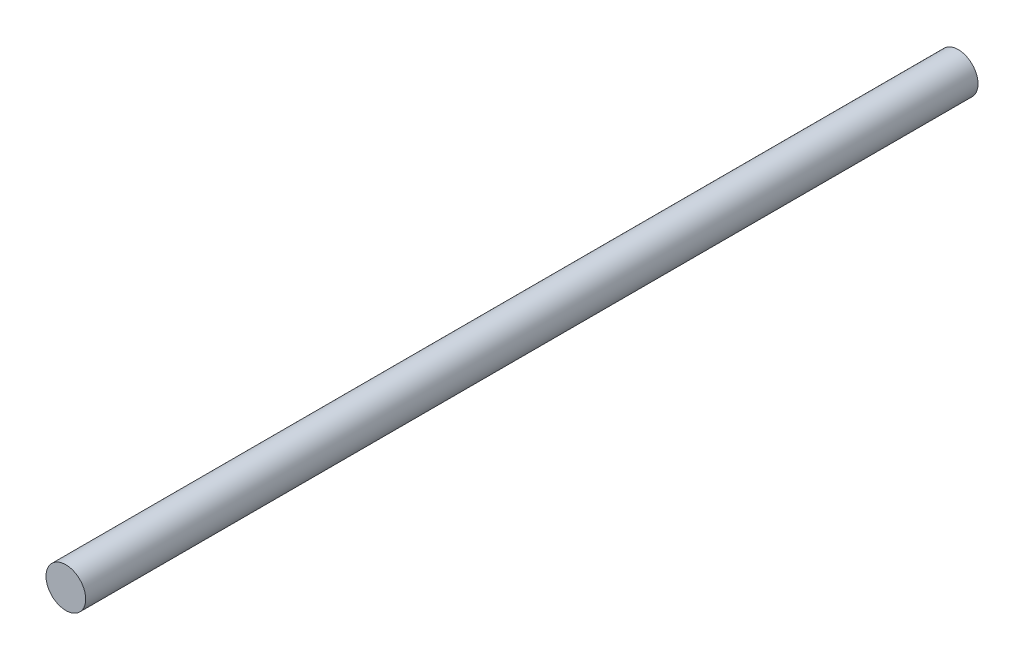
from build123d import *

# Parameters (mm, degrees)
SKETCH1_R           = 2
BOSS_EXTRUDE1_DEPTH = 90


with BuildPart() as part:
    # Sketch1 → Boss-Extrude1 (new body)
    with BuildSketch(Plane.XY):
        with Locations(Location((0, 0, 0), (0, 0, 180))):
            Circle(SKETCH1_R)
    extrude(amount=BOSS_EXTRUDE1_DEPTH)


solid = part.part
